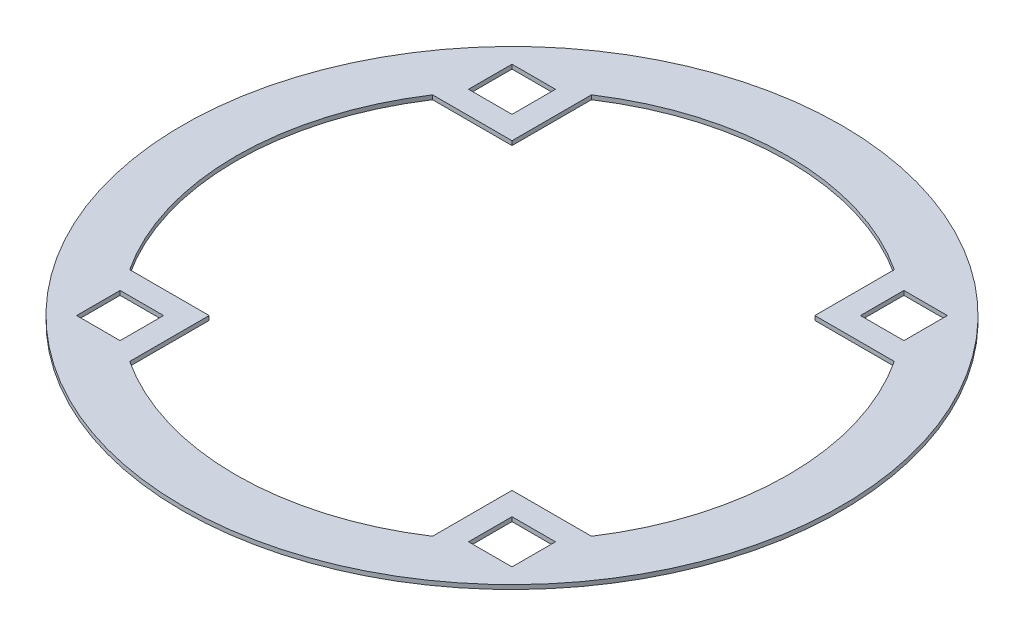
SolidWorks part; units mm, degrees
material "XRAAT"
ref_plane "前视基准面" through (0, 0, 0) normal (0, 0, 1) x (1, 0, 0)
ref_plane "上视基准面" through (0, 0, 0) normal (0, 1, 0) x (1, 0, 0)
ref_plane "右视基准面" through (0, 0, 0) normal (1, 0, 0) x (0, 0, -1)
sketch "草图1" plane through (0, 0, 0) normal (0, 1, 0) x (1, 0, 0)
  line L0 (-425, 425) -> (-425, 648.0741)
  line L1 (425, -425) -> (-425, -425)
  line L2 (425, -425) -> (425, 425)
  line L3 (425, 425) -> (-425, 425)
  line L4 (-425, -425) -> (-425, 425)
  line L5 (425, -425) -> (-425, 425) construction
  line L6 (425, 425) -> (-425, -425) construction
  line L7 (-425, 425) -> (-648.0741, 425)
  line L8 (-425, 0) -> (0, 0) construction
  line L9 (0, 0) -> (0, 425) construction
  line L10 (-425, -425) -> (-425, -648.0741)
  line L11 (-425, -425) -> (-648.0741, -425)
  line L12 (425, -425) -> (425, -648.0741)
  line L13 (425, -425) -> (648.0741, -425)
  line L14 (425, 425) -> (648.0741, 425)
  line L15 (425, 425) -> (425, 648.0741)
  line L16 (489, 611) -> (611, 489) construction
  line L17 (-489, 489) -> (-611, 489)
  line L18 (-489, 489) -> (-489, 611)
  line L19 (-489, 611) -> (-611, 611)
  line L20 (-611, 489) -> (-611, 611)
  line L21 (-489, 489) -> (-611, 611) construction
  line L22 (-489, 611) -> (-611, 489) construction
  line L23 (489, 489) -> (611, 611) construction
  line L24 (611, 489) -> (611, 611)
  line L25 (489, 611) -> (611, 611)
  line L26 (489, 489) -> (489, 611)
  line L27 (489, 489) -> (611, 489)
  line L28 (489, -489) -> (611, -611) construction
  line L29 (489, -611) -> (611, -489) construction
  line L30 (489, -489) -> (611, -489)
  line L31 (489, -489) -> (489, -611)
  line L32 (489, -611) -> (611, -611)
  line L33 (611, -489) -> (611, -611)
  line L34 (-489, -611) -> (-611, -489) construction
  line L35 (-489, -489) -> (-611, -611) construction
  line L36 (-611, -489) -> (-611, -611)
  line L37 (-489, -611) -> (-611, -611)
  line L38 (-489, -489) -> (-489, -611)
  line L39 (-489, -489) -> (-611, -489)
  circle A0 centre (0, 0) radius 925
  circle A1 centre (0, 0) radius 775
  point P18 (-550, 550)
  point P28 (550, 550)
  point P33 (550, -550)
  point P38 (-550, -550)
  dimension "D1" = 1850
  dimension "D2" = 1550
  dimension "D3" = 850
  dimension "D4" = 122
  dimension "D5" = 1100
  dimension "D6" = 1100
extrude "凸台-拉伸1" add sketch "草图1" along normal blind 12 contours A0 A1 L30 L33 L32 L31 L38 L37 L36 L39 L17 L20 L19 L18 L26 L25 L24 L27 | L30 A1 L13 L12 L31 | L11 A1 L39 L38 L10 | L0 A1 L18 L17 L7 | L14 A1 L27 L26 L15
